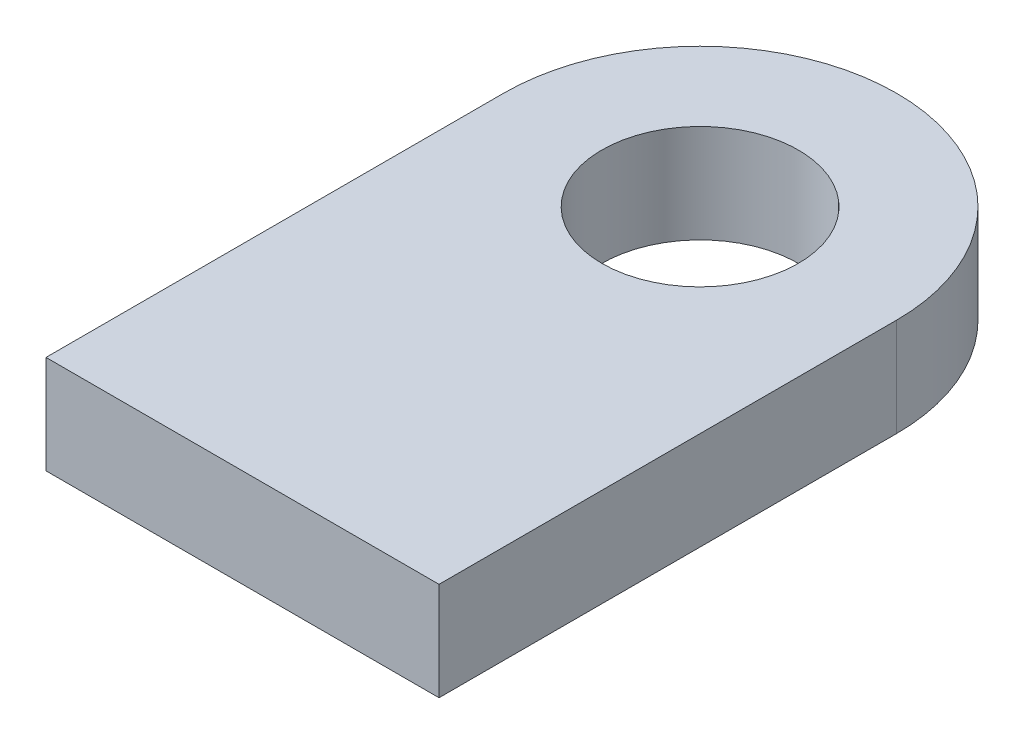
from build123d import *

# Parameters (mm, degrees)
SKETCH_1_R      = 10
EXTRUDE_1_DEPTH = 5


with BuildPart() as part:
    # 草图1 → 凸台-拉伸1 (new, symmetric)
    with BuildSketch(Plane(origin=(0, 0, 0), x_dir=(1, 0, 0), z_dir=(0, 1, 0))):
        with BuildLine():
            Line((-20, -23.285), (20, -23.285))
            Line((20, -23.285), (20, 23.285))
            ThreePointArc((20, 23.285), (0, 43.285), (-20, 23.285))
            Line((-20, 23.285), (-20, -23.285))
        make_face()
        with Locations(Location((0, 23.285, 0), (0, 0, 270))):
            Circle(SKETCH_1_R, mode=Mode.SUBTRACT)
    extrude(amount=EXTRUDE_1_DEPTH, both=True)


solid = part.part
